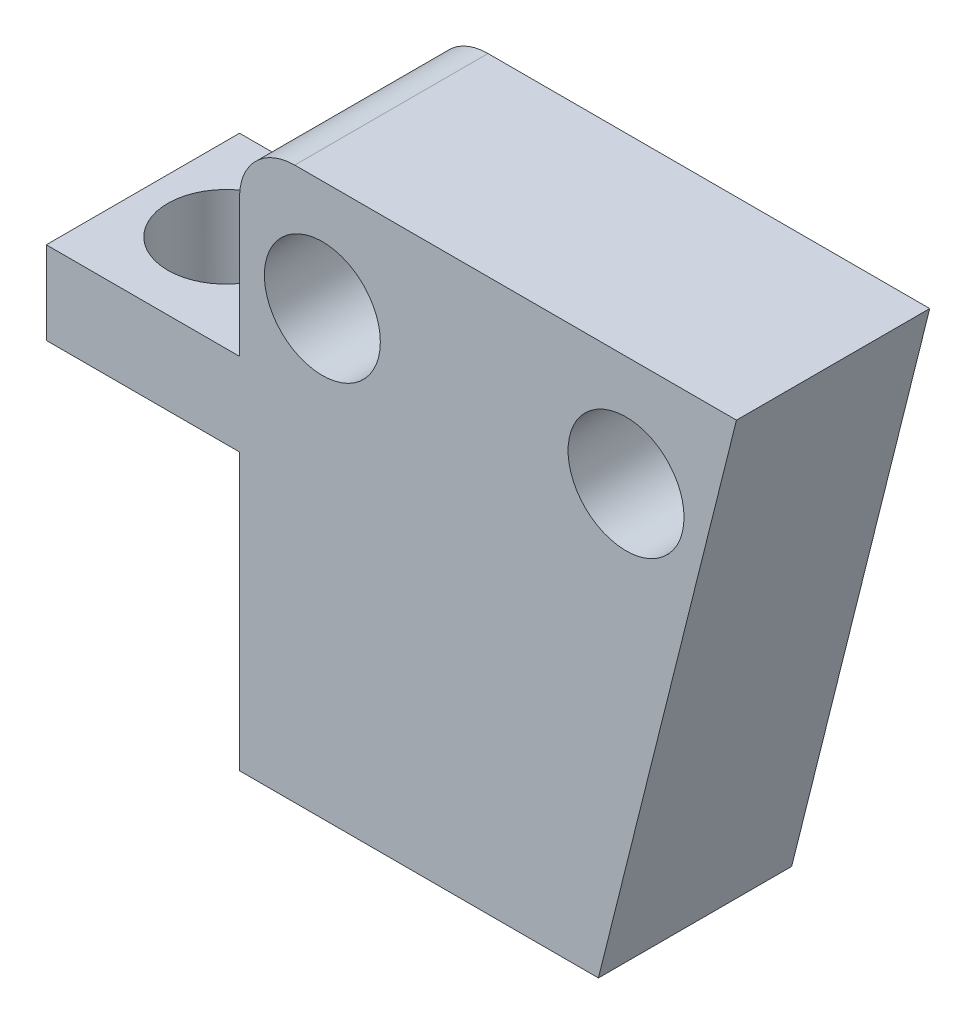
SolidWorks part; units mm, degrees
ref_plane "Front Plane" through (0, 0, 0) normal (0, 0, 1) x (1, 0, 0)
ref_plane "Top Plane" through (0, 0, 0) normal (0, 1, 0) x (1, 0, 0)
ref_plane "Right Plane" through (0, 0, 0) normal (1, 0, 0) x (0, 0, -1)
sketch "Sketch2" plane through (0, 0, 0) normal (0, 0, 1) x (1, 0, 0)
  line L0 (0, 0) -> (0, 12.7)
  line L1 (0, 12.7) -> (-8.89, 12.7)
  line L2 (-8.89, 12.7) -> (-8.89, 16.51)
  line L3 (-8.89, 16.51) -> (0, 16.51)
  line L4 (0, 16.51) -> (0, 25.4)
  line L5 (0, 25.4) -> (22.86, 25.4)
  line L6 (22.86, 25.4) -> (16.51, 0)
  line L7 (16.51, 0) -> (0, 0)
  circle A0 centre (3.81, 20.32) radius 2.667
  circle A1 centre (17.78, 20.32) radius 2.667
  dimension "D1" = 5.334
  dimension "D2" = 5.334
  dimension "D7" = 20.32
  dimension "D3" = 13.97
  dimension "D4" = 22.86
  dimension "D5" = 3.81
  dimension "D6" = 20.32
  dimension "D8" = 25.4
  dimension "D9" = 16.51
  dimension "D10" = 12.7
  dimension "D11" = 3.81
  dimension "D12" = 8.89
extrude "Boss-Extrude1" add sketch "Sketch2" along normal blind 8.89
sketch "Sketch3" plane through (0, 16.51, 0) normal (0, 1, 0) x (1, 0, 0)
  line L0 (0, -8.89) -> (0, 0) construction
  line L2 (-5.08, -4.445) -> (-8.89, -4.445) construction
  line L3 (-8.89, -8.89) -> (-8.89, 0) construction
  circle A0 centre (-5.08, -4.445) radius 2.667
  dimension "D2" = 5.334
  dimension "D1" = 5.08
extrude "Cut-Extrude1" cut sketch "Sketch3" against normal through all
fillet "Fillet1" radius 2.54 1 edges at (0, 25.4, 4.445)
scale "Scale1" bodies to scale 102 scale about origin uniform scaling yes scale factor 2
